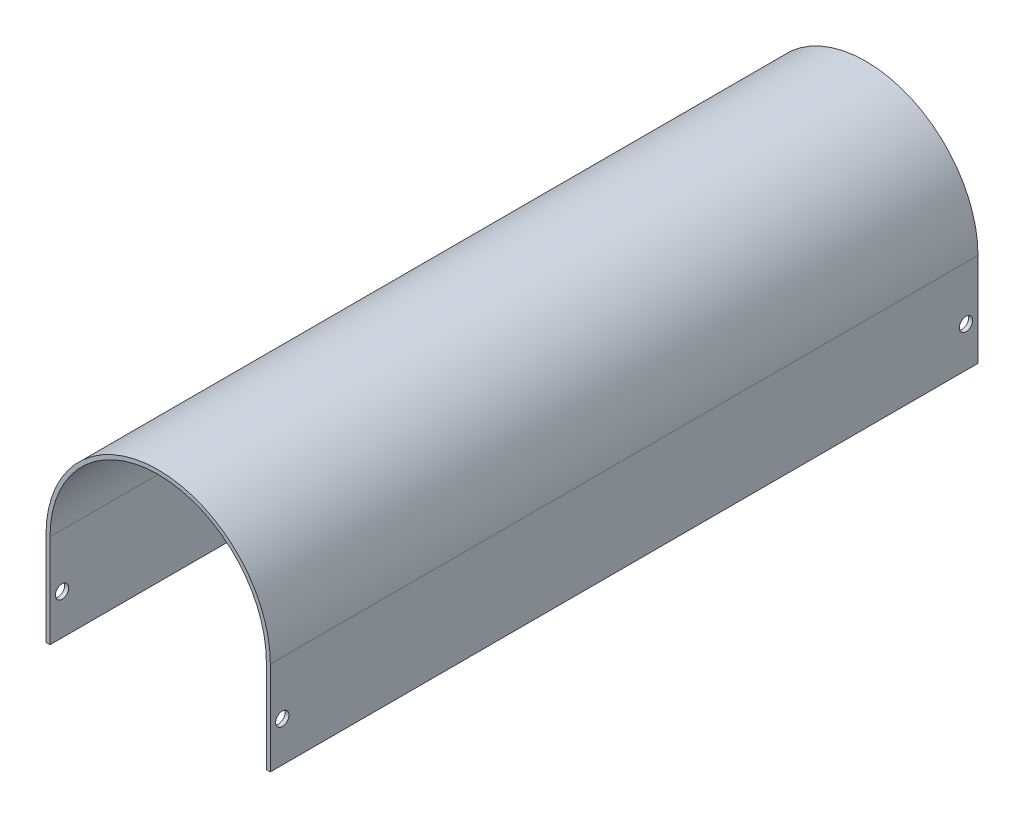
from build123d import *

# Parameters (mm, degrees)
EXTRUDE_1_DEPTH     = 265
SKETCH_2_R          = 2.5
CUT_EXTRUDE_1_DEPTH = 289.461435897


with BuildPart() as part:
    # 草图1 → 凸台-拉伸1 (new body)
    with BuildSketch(Plane.XY):
        with BuildLine():
            Line((-20.582221357, 0), (-19.082221357, 0))
            Line((-19.082221357, 0), (-19.082221357, 35))
            ThreePointArc((-19.082221357, 35), (21.417778643, 75.5), (61.917778643, 35))
            Line((61.917778643, 35), (61.917778643, 0))
            Line((61.917778643, 0), (63.417778643, 0))
            Line((63.417778643, 0), (63.417778643, 35))
            ThreePointArc((63.417778643, 35), (21.417778643, 77), (-20.582221357, 35))
            Line((-20.582221357, 35), (-20.582221357, 0))
        make_face()
    extrude(amount=EXTRUDE_1_DEPTH)

    # 草图2 → 切除-拉伸1 (cut, through all)
    with BuildSketch(Plane(origin=(63.417778643, 0, 0), x_dir=(0, 0, -1), z_dir=(1, 0, 0))):
        with Locations(Location((-260.5, 15, 0), (0, 0, 90))):
            Circle(SKETCH_2_R)
        with Locations(Location((-4.5, 15, 0), (0, 0, 90))):
            Circle(SKETCH_2_R)
    extrude(amount=-CUT_EXTRUDE_1_DEPTH, mode=Mode.SUBTRACT)


solid = part.part
